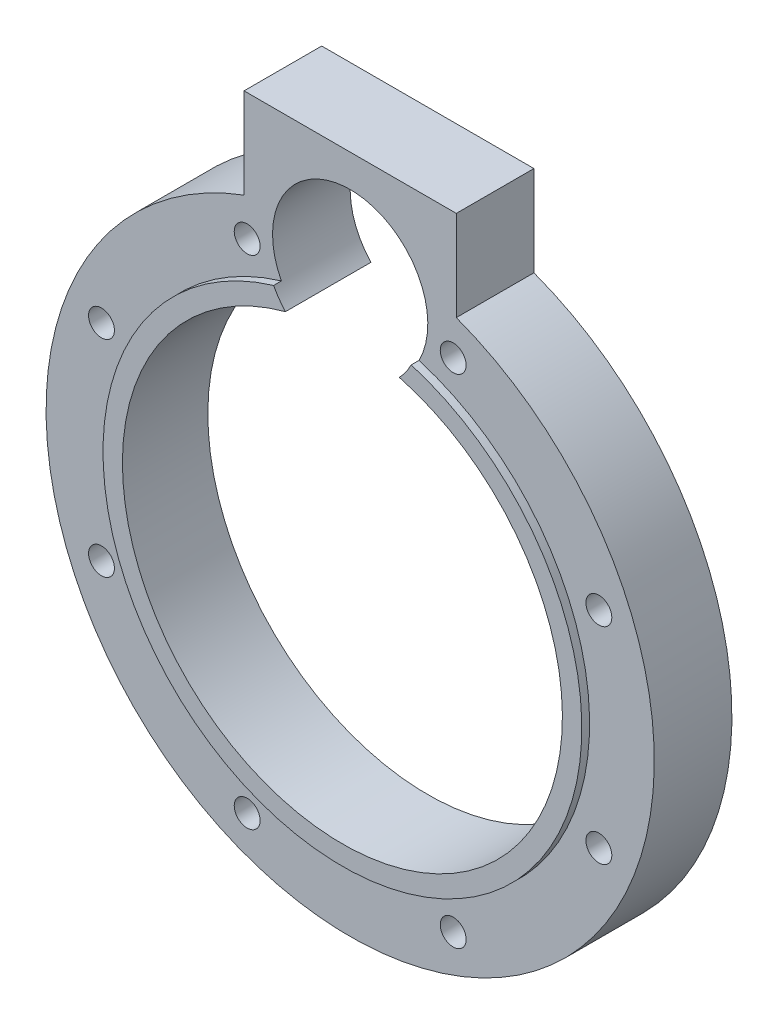
SolidWorks part; units mm, degrees
material "Q235A"
ref_plane "前视基准面" through (0, 0, 0) normal (0, 0, 1) x (1, 0, 0)
ref_plane "上视基准面" through (0, 0, 0) normal (0, 1, 0) x (1, 0, 0)
ref_plane "右视基准面" through (0, 0, 0) normal (1, 0, 0) x (0, 0, -1)
sketch "草图1" plane through (0, 0, 0) normal (0, 0, 1) x (1, 0, 0)
  line L0 (0, 0) -> (0, 166.7324) construction
  circle A0 centre (0, 0) radius 85
  circle A1 centre (0, 0) radius 117.5
  dimension "D1" = 170
  dimension "D2" = 235
extrude "凸台-拉伸1" add sketch "草图1" along normal blind 30
sketch "草图3" plane through (0, 0, 30) normal (0, 0, 1) x (1, 0, 0)
  line L0 (0, 0) -> (0, 115) construction
  line L2 (-41, 85) -> (41, 85)
  line L3 (-41, 85) -> (-41, 145)
  line L4 (-41, 145) -> (41, 145)
  line L5 (41, 85) -> (41, 145)
  line L6 (-41, 85) -> (41, 145) construction
  line L7 (-41, 145) -> (41, 85) construction
  circle A0 centre (0, 0) radius 85 construction
  dimension "D1" = 82
  dimension "D2" = 145
extrude "凸台-拉伸5" add sketch "草图3" against normal through all
hole_wizard "M8 间隙孔1" positions "草图5" profile "草图6" hole size "M8" standard "ISO" end condition through all
sketch "草图5" plane through (0, 0, 0) normal (0, 0, -1) x (-1, 0, 0)
  line L4 (0, 0) -> (0, 152.9093) construction
  line L6 (-39.7991, 96.0835) -> (0, 0) construction
  point P0 (-39.7991, 96.0835)
  point P11 (39.7991, 96.0835)
  point P12 (96.0835, 39.7991)
  point P13 (96.0835, -39.7991)
  point P14 (39.7991, -96.0835)
  point P15 (-39.7991, -96.0835)
  point P16 (-96.0835, -39.7991)
  point P17 (-96.0835, 39.7991)
  dimension "D1" = 104
  dimension "D3" = 208
  dimension "D2" = 8
sketch "草图6" plane through (39.7991, 96.0835, 0) normal (1, 0, 0) x (0, 1, 0)
  line L0 (0, 0) -> (0, 30)
  line L1 (0, 30) -> (5, 30)
  line L2 (5, 30) -> (5, 0)
  line L5 (5, 0) -> (0, 0)
  line L11 (0, -6.35) -> (0, 107.95) construction
  dimension "通孔孔直径" = 10
  dimension "通孔孔深度" = 30
sketch "草图9" plane through (0, 0, 30) normal (0, 0, 1) x (1, 0, 0)
  circle A0 centre (0, 0) radius 92.5
  circle A1 centre (0, 0) radius 85 construction
  circle A2 centre (0, 0) radius 85
  dimension "D1" = 185
extrude "凸台-拉伸7" add sketch "草图9" along normal blind 3
sketch "草图8" plane through (0, 0, 0) normal (0, 0, -1) x (-1, 0, 0)
  circle A0 centre (0, 102.5) radius 30
  dimension "D1" = 60
extrude "切除-拉伸1" cut sketch "草图8" against normal through all
